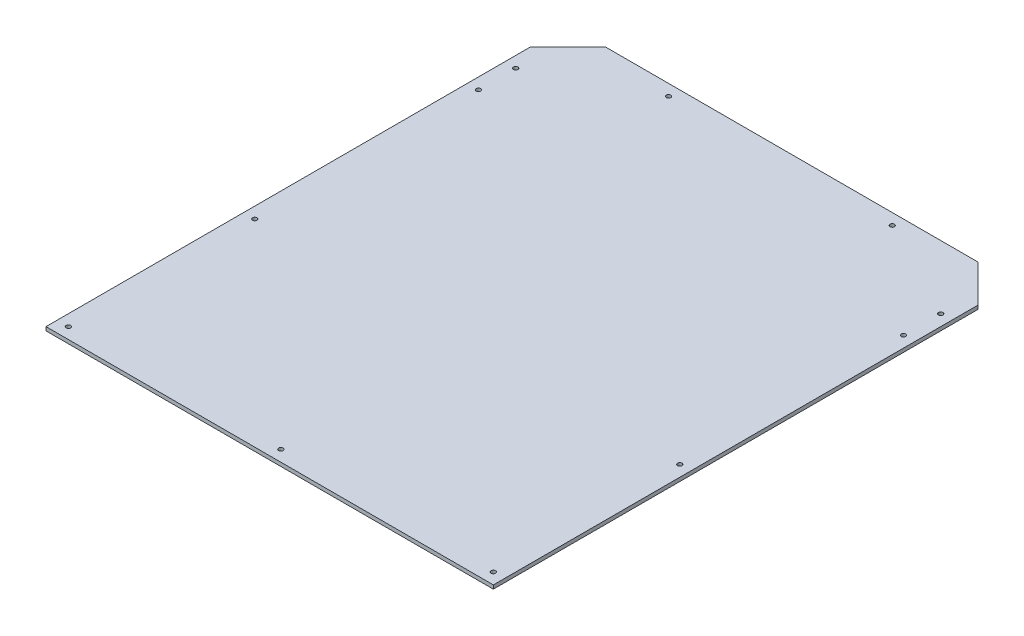
from build123d import *

# Parameters (mm, degrees)
EXTRUDE_1_DEPTH     = 5
SKETCH_2_R          = 3
CUT_EXTRUDE_1_DEPTH = 10


with BuildPart() as part:
    # 草图1 → 凸台-拉伸1 (new body)
    with BuildSketch(Plane(origin=(0, 0, 0), x_dir=(1, 0, 0), z_dir=(0, 1, 0))):
        Polygon((0, 650), (50, 700), (550, 700), (600, 650), (600, 0), (0, 0), align=None)
    extrude(amount=EXTRUDE_1_DEPTH)

    # 草图2 → 切除-拉伸1 (cut)
    with BuildSketch(Plane(origin=(0, 5, 0), x_dir=(1, 0, 0), z_dir=(0, 1, 0))):
        with Locations(Location((15, 15, 0), (0, 0, 270))):
            Circle(SKETCH_2_R)
        with Locations(Location((15, 265, 0), (0, 0, 270))):
            Circle(SKETCH_2_R)
        with Locations(Location((15, 565, 0), (0, 0, 270))):
            Circle(SKETCH_2_R)
        with Locations(Location((15, 615, 0), (0, 0, 270))):
            Circle(SKETCH_2_R)
        with Locations(Location((150, 685, 0), (0, 0, 270))):
            Circle(SKETCH_2_R)
        with Locations(Location((585, 15, 0), (0, 0, 90))):
            Circle(SKETCH_2_R)
        with Locations(Location((585, 265, 0), (0, 0, 90))):
            Circle(SKETCH_2_R)
        with Locations(Location((585, 565, 0), (0, 0, 90))):
            Circle(SKETCH_2_R)
        with Locations(Location((585, 615, 0), (0, 0, 90))):
            Circle(SKETCH_2_R)
        with Locations(Location((450, 685, 0), (0, 0, 90))):
            Circle(SKETCH_2_R)
        with Locations(Location((300, 15, 0), (0, 0, 270))):
            Circle(SKETCH_2_R)
    extrude(amount=-CUT_EXTRUDE_1_DEPTH, mode=Mode.SUBTRACT)


solid = part.part
